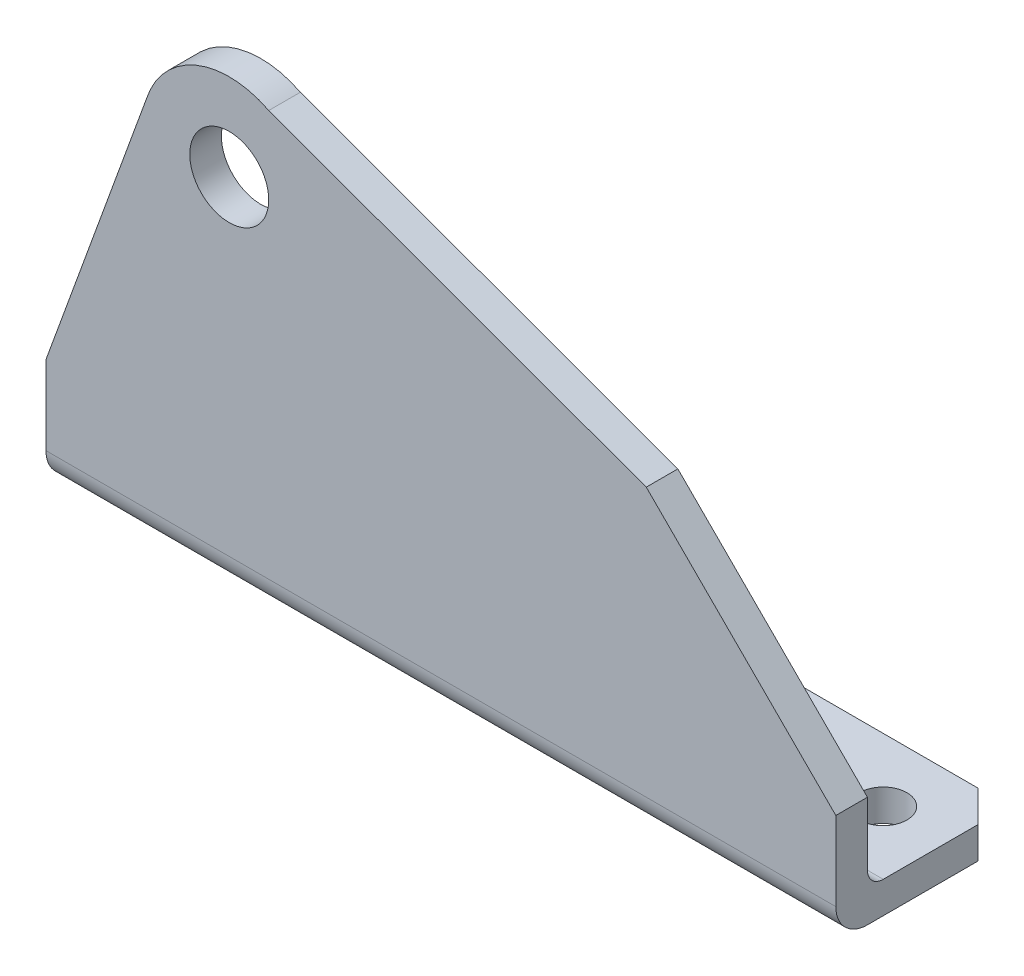
from build123d import *

# Parameters (mm, degrees)
SKETCH1_W           = 250
SKETCH1_H           = 181
BOSS_EXTRUDE1_DEPTH = 10
SKETCH2_OUTSIDE_W   = 313.762
SKETCH2_OUTSIDE_H   = 244.762
CUT_EXTRUDE1_DEPTH  = 10
SKETCH3_R           = 12.5
CUT_EXTRUDE2_DEPTH  = 10
SKETCH4_W           = 250
SKETCH4_H           = 10
BOSS_EXTRUDE2_DEPTH = 45
FILLET1_R           = 10
FILLET2_R           = 5
SKETCH5_R           = 7.5
CUT_EXTRUDE3_DEPTH  = 45
CHAMFER1_SIZE       = 10


with BuildPart() as part:
    # Sketch1 → Boss-Extrude1 (new body)
    with BuildSketch(Plane.XY):
        Rectangle(SKETCH1_W, SKETCH1_H)
    extrude(amount=BOSS_EXTRUDE1_DEPTH)

    # Sketch2 outside → Cut-Extrude1 (cut)
    with BuildSketch(Plane.XY.offset(10)):
        Rectangle(SKETCH2_OUTSIDE_W, SKETCH2_OUTSIDE_H)
        with BuildLine():
            Line((-125, -55.5), (-93.159896838, 31.97996447))
            ThreePointArc((-93.159896838, 31.97996447), (-77.523014584, 48.907010136), (-54.496896373, 47.993313367))
            Line((-54.496896373, 47.993313367), (65, 4.5))
            Line((65, 4.5), (125, -55.5))
            Line((125, -55.5), (125, -90.5))
            Line((125, -90.5), (-125, -90.5))
            Line((-125, -90.5), (-125, -55.5))
        make_face(mode=Mode.SUBTRACT)
    extrude(amount=-CUT_EXTRUDE1_DEPTH, mode=Mode.SUBTRACT)

    # Sketch3 → Cut-Extrude2 (cut)
    with BuildSketch(Plane.XY.offset(10)):
        with Locations((-67, 23.5)):
            Circle(SKETCH3_R)
    extrude(amount=-CUT_EXTRUDE2_DEPTH, mode=Mode.SUBTRACT)

    # Sketch4 → Boss-Extrude2 (add)
    with BuildSketch(Plane(origin=(0, 0, 0), x_dir=(-1, 0, 0), z_dir=(0, 0, -1))):
        with Locations((0, -85.5)):
            Rectangle(SKETCH4_W, SKETCH4_H)
    extrude(amount=BOSS_EXTRUDE2_DEPTH)

    # Fillet1
    fillet1_edges = [part.edges().sort_by_distance(p)[0] for p in [
        (0, -90.5, 10),
    ]]
    fillet(fillet1_edges, radius=FILLET1_R)

    # Fillet2
    fillet2_edges = [part.edges().sort_by_distance(p)[0] for p in [
        (0, -80.5, 0),
    ]]
    fillet(fillet2_edges, radius=FILLET2_R)

    # Sketch5 → Cut-Extrude3 (cut)
    with BuildSketch(Plane.XZ.offset(90.5)):
        with Locations((-105, -25)):
            Circle(SKETCH5_R)
        with Locations((105, -25)):
            Circle(SKETCH5_R)
    extrude(amount=-CUT_EXTRUDE3_DEPTH, mode=Mode.SUBTRACT)

    # Chamfer1
    chamfer1_edges = [part.edges().sort_by_distance(p)[0] for p in [
        (125, -85.5, -45),
        (-125, -85.5, -45),
    ]]
    chamfer(chamfer1_edges, length=CHAMFER1_SIZE)


solid = part.part
